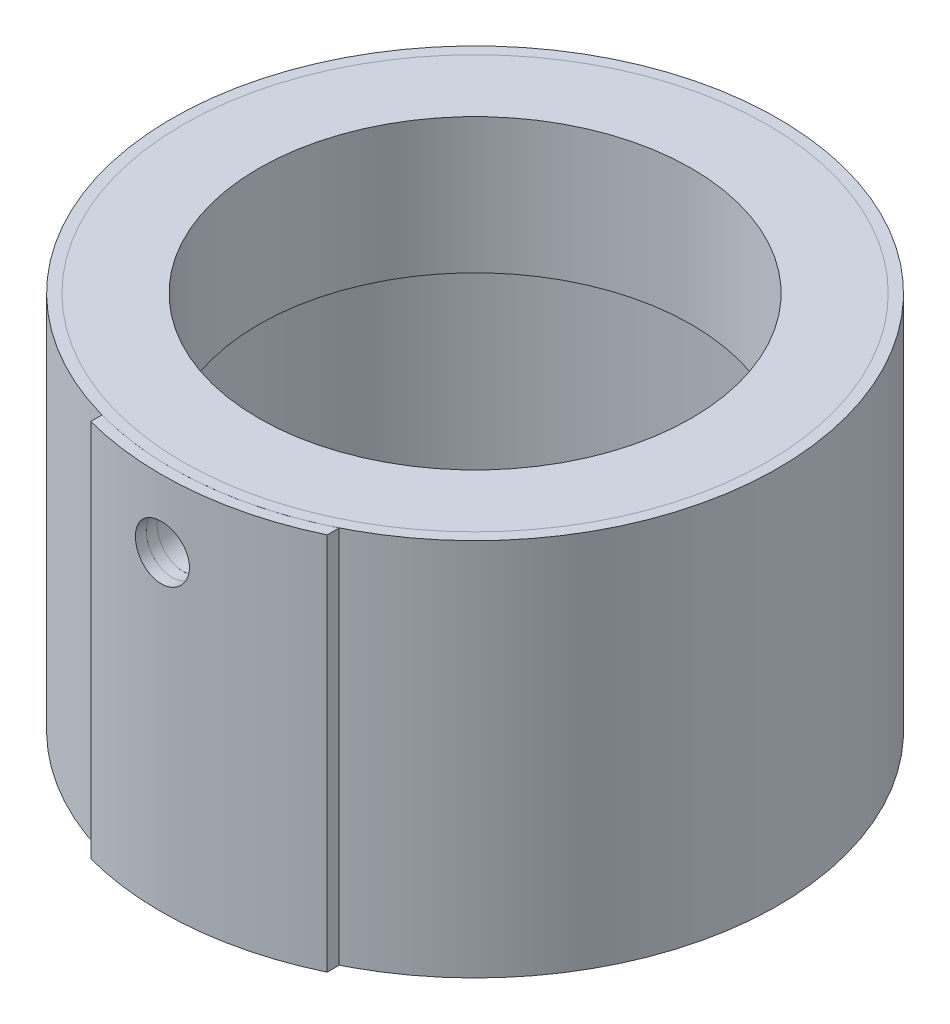
from build123d import *

# Parameters (mm, degrees)
SKETCH_1_R          = 54
SKETCH_1_R_2        = 40
EXTRUDE_1_DEPTH     = 25
SKETCH_2_R          = 56
SKETCH_2_R_2        = 54
EXTRUDE_2_DEPTH     = 70
EXTRUDE_3_DEPTH     = 70
SKETCH_3_R          = 5
CUT_EXTRUDE_1_DEPTH = 93.330926563


with BuildPart() as part:
    # 草图1 → 凸台-拉伸1 (new body)
    with BuildSketch(Plane(origin=(0, 0, 0), x_dir=(1, 0, 0), z_dir=(0, 1, 0))):
        with Locations(Location((0, 0, 0), (0, 0, 270))):
            Circle(SKETCH_1_R)
        with Locations(Location((0, 0, 0), (0, 0, 270))):
            Circle(SKETCH_1_R_2, mode=Mode.SUBTRACT)
    extrude(amount=EXTRUDE_1_DEPTH)


with BuildPart() as body_2:
    # 草图2 → 凸台-拉伸2 (new body)
    with BuildSketch(Plane(origin=(0, 25, 0), x_dir=(1, 0, 0), z_dir=(0, 1, 0))):
        with Locations(Location((0, 0, 0), (0, 0, 270))):
            Circle(SKETCH_2_R)
        with Locations(Location((0, 0, 0), (0, 0, 270))):
            Circle(SKETCH_2_R_2, mode=Mode.SUBTRACT)
    extrude(amount=-EXTRUDE_2_DEPTH)


with BuildPart() as body_3:
    # 草图4 → 凸台-拉伸3 (new body)
    with BuildSketch(Plane(origin=(0, 25, 0), x_dir=(1, 0, 0), z_dir=(0, 1, 0))):
        with BuildLine():
            Line((25, -50.109879265), (25, -52.335456433))
            ThreePointArc((25, -52.335456433), (5.329771679, -57.754597513), (-15, -56.026779311))
            Line((-15, -56.026779311), (-15, -53.953683841))
            ThreePointArc((-15, -53.953683841), (5.356650857, -55.743217449), (25, -50.109879265))
        make_face()
    extrude(amount=-EXTRUDE_3_DEPTH)


with BuildPart() as cut_extrude_1_tool:
    # 草图3 → 切除-拉伸1 (new, through all)
    with BuildSketch(Plane.XY):
        with Locations(Location((0, 12.5, 0), (0, 0, 180))):
            Circle(SKETCH_3_R)
    extrude(amount=CUT_EXTRUDE_1_DEPTH)


with BuildPart() as part_1:
    add(part.part)

    # 切除-拉伸1: cut by cut_extrude_1_tool
    add(cut_extrude_1_tool.part, mode=Mode.SUBTRACT)


with BuildPart() as body_2_1:
    add(body_2.part)

    # 切除-拉伸1: cut by cut_extrude_1_tool
    add(cut_extrude_1_tool.part, mode=Mode.SUBTRACT)


with BuildPart() as body_3_1:
    add(body_3.part)

    # 切除-拉伸1: cut by cut_extrude_1_tool
    add(cut_extrude_1_tool.part, mode=Mode.SUBTRACT)


solid = Compound([part_1.part, body_2_1.part, body_3_1.part])
